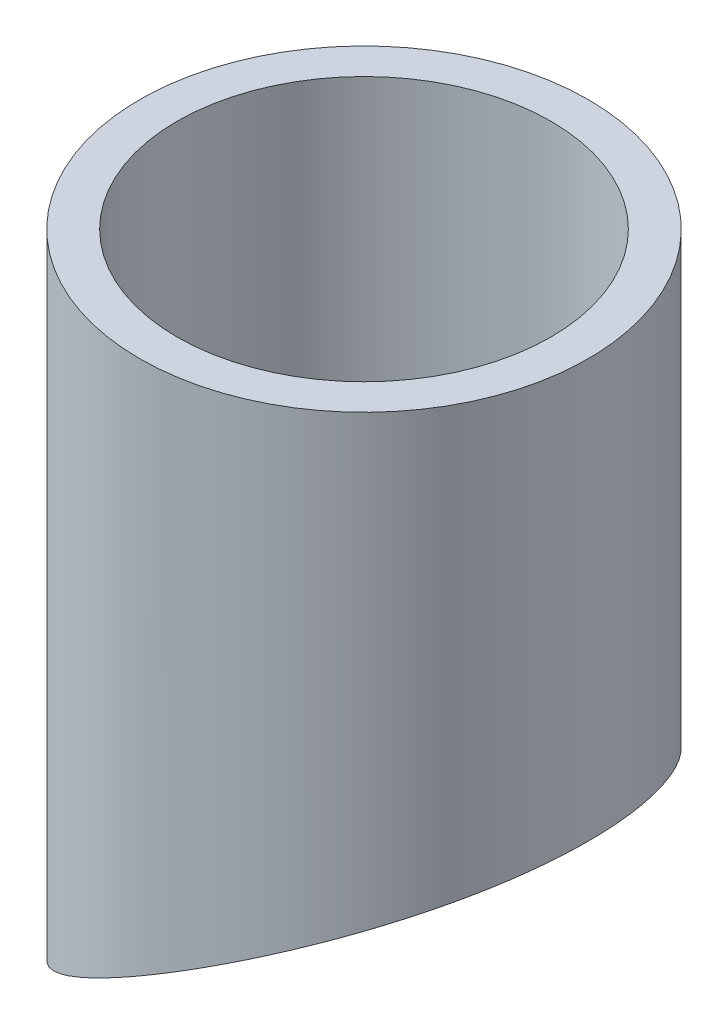
SolidWorks part; units mm, degrees
material "不锈钢管60×5"
ref_plane "Front Plane" through (0, 0, 0) normal (0, 0, 1) x (1, 0, 0)
ref_plane "Top Plane" through (0, 0, 0) normal (0, 1, 0) x (1, 0, 0)
ref_plane "Right Plane" through (0, 0, 0) normal (1, 0, 0) x (0, 0, -1)
sketch "Sketch2" plane through (0, 0, 0) normal (0, 1, 0) x (1, 0, 0)
  circle A0 centre (0, 0) radius 30
  circle A1 centre (0, 0) radius 25
  dimension "D1" = 60
  dimension "D2" = 50
extrude "Boss-Extrude1" add sketch "Sketch2" along normal blind 400
cosmetic thread "Cosmetic Thread1" parameters "D1"=25, "D2"=56.656
sketch "Sketch3" plane through (0, 0, 0) normal (0, 0, 1) x (1, 0, 0)
  line L0 (0, 0) -> (190, 0) construction
  circle A2 centre (190, 0) radius 379.5
  dimension "D1" = 759
  dimension "D2" = 190
extrude "Cut-Extrude1" cut sketch "Sketch3" against normal through all both and the other way through all
